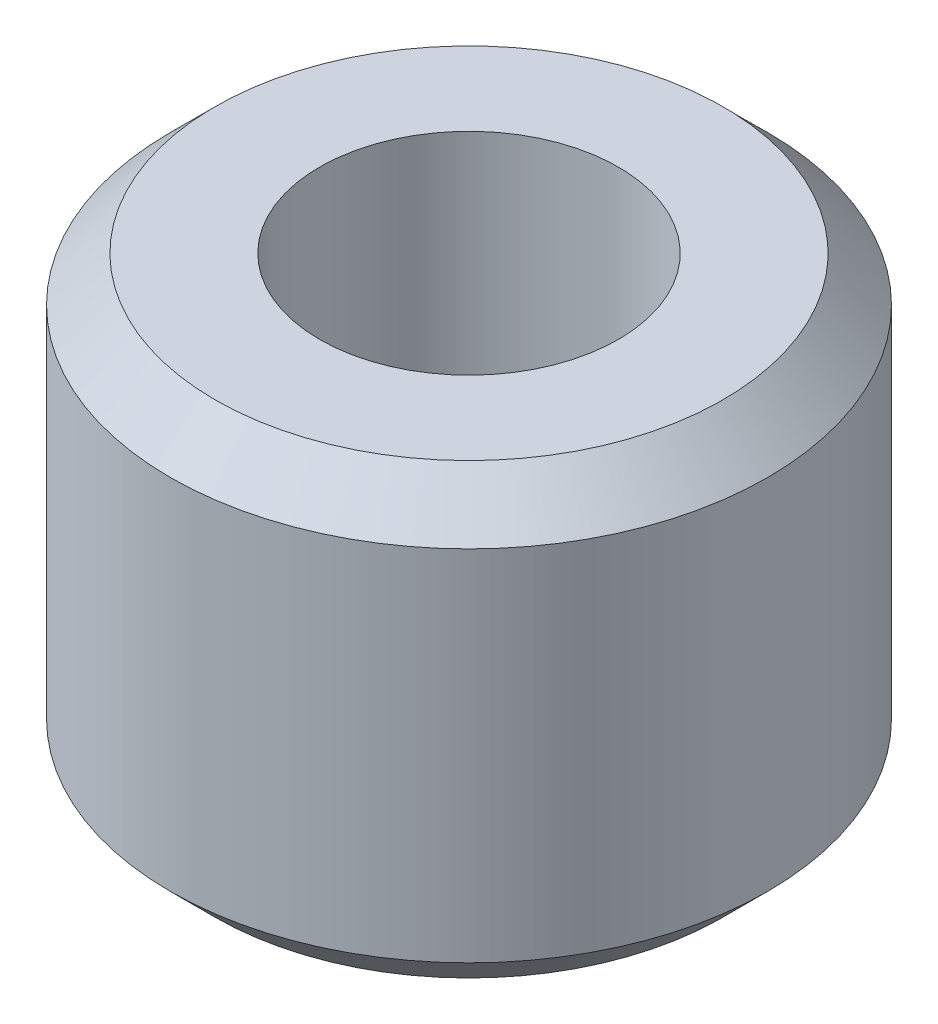
from build123d import *

# Parameters (mm, degrees)
SKETCH1_R           = 20
SKETCH1_R_2         = 10
BOSS_EXTRUDE1_DEPTH = 30
CHAMFER1_SIZE       = 3


with BuildPart() as part:
    # Sketch1 → Boss-Extrude1 (new body)
    with BuildSketch(Plane(origin=(0, 0, 0), x_dir=(1, 0, 0), z_dir=(0, 1, 0))):
        with Locations(Location((0, 0, 0), (0, 0, 270))):
            Circle(SKETCH1_R)
        with Locations(Location((0, 0, 0), (0, 0, 270))):
            Circle(SKETCH1_R_2, mode=Mode.SUBTRACT)
    extrude(amount=BOSS_EXTRUDE1_DEPTH)

    # Chamfer1
    chamfer1_edges = [part.edges().sort_by_distance(p)[0] for p in [
        (0, 0, -20),
        (0, 30, -20),
    ]]
    chamfer(chamfer1_edges, length=CHAMFER1_SIZE)


solid = part.part
